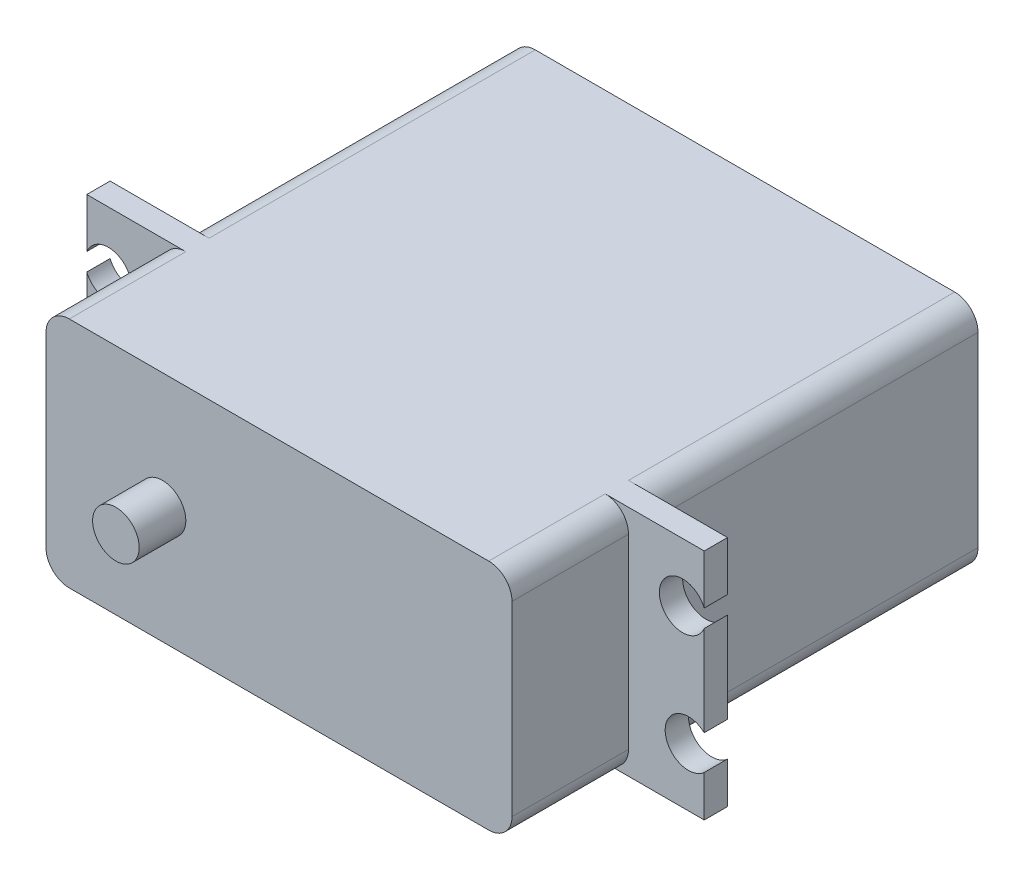
SolidWorks part; units mm, degrees
ref_plane "Front Plane" through (0, 0, 0) normal (0, 0, 1) x (1, 0, 0)
ref_plane "Top Plane" through (0, 0, 0) normal (0, 1, 0) x (1, 0, 0)
ref_plane "Right Plane" through (0, 0, 0) normal (1, 0, 0) x (0, 0, -1)
sketch "Sketch1" plane through (0, 0, 0) normal (0, 1, 0) x (1, 0, 0)
  line L1 (-20, -20) -> (20, -20)
  line L2 (-20, -20) -> (-20, 20)
  line L3 (-20, 20) -> (20, 20)
  line L4 (20, -20) -> (20, 20)
  line L5 (-20, -20) -> (20, 20) construction
  line L6 (-20, 20) -> (20, -20) construction
  point P0 (0, 0)
  dimension "D1" = 40
  dimension "D2" = 40
extrude "Boss-Extrude1" add sketch "Sketch1" along normal blind 20
ref_plane "Plane1" through (0, 0, 8) normal (0, 0, -1) x (-1, 0, 0)
sketch "Sketch2" plane through (0, 0, 8) normal (0, 0, -1) x (-1, 0, 0)
  line L0 (26.5, 0) -> (26.5, 20)
  line L2 (-26.5, 20) -> (-26.5, 0)
  line L4 (-20, 0) -> (20, 0)
  line L5 (20, 0) -> (20, 20)
  line L6 (20, 20) -> (-20, 20)
  line L7 (-20, 20) -> (-20, 0)
  line L8 (-20, 0) -> (20, 0)
  line L9 (20, 0) -> (20, 20)
  line L10 (20, 20) -> (-20, 20)
  line L11 (-20, 20) -> (-20, 0)
  line L12 (20, 0) -> (26.5, 0)
  line L13 (20, 20) -> (26.5, 20)
  line L14 (-20, 0) -> (-26.5, 0)
  line L15 (-20, 20) -> (-26.5, 20)
  line L16 (-26.5, 26.5) -> (-26.5, -6.5) construction
  line L17 (26.5, 26.5) -> (-26.5, 26.5) construction
  line L18 (26.5, -6.5) -> (26.5, 26.5) construction
  line L19 (-26.5, -6.5) -> (26.5, -6.5) construction
  dimension "D1" = 0
  dimension "D2" = 6.5
extrude "Boss-Extrude2" add sketch "Sketch2" against normal blind 2 contours L13 L9 L12 L0 | L11 L15 L2 L14
sketch "Sketch3" plane through (0, 0, 8) normal (0, 0, -1) x (-1, 0, 0)
  line L0 (20, 20) -> (26.5, 20) construction
  line L1 (26.5, 0) -> (26.5, 20) construction
  circle A0 centre (25.1494, 5.0125) radius 2
  circle A1 centre (24.65, 15) radius 2
  dimension "D2" = 4
  dimension "D3" = 4
  dimension "D1" = 10
  dimension "D4" = 5
  dimension "D5" = 1.85
extrude "Cut-Extrude1" cut sketch "Sketch3" against normal blind 2
ref_plane "Plane2" through (0, 0, 0) normal (-1, 0, 0) x (0, 0, 1)
mirror "Mirror2" about plane through (0, 0, 0) normal (-1, 0, 0) of "Cut-Extrude1"
sketch "Sketch4" plane through (0, 0, 20) normal (0, 0, 1) x (1, 0, 0)
  line L0 (20, 20) -> (20, 0) construction
  circle A0 centre (-10, 10) radius 2
  dimension "D2" = 4
  dimension "D1" = 30
extrude "Boss-Extrude3" add sketch "Sketch4" along normal blind 4
fillet "Fillet1" radius 2 8 edges
sketch "Sketch5" plane through (0, 0, 20) normal (0, 0, 1) x (1, 0, 0)
  line L0 (-10, 10) -> (-10, 20) construction
  line L1 (-18, 20) -> (18, 20) construction
sketch "Sketch6" plane through (0, 0, 0) normal (0, 1, 0) x (1, 0, 0)
  line L0 (-10, -20) -> (-10, 20) construction
  line L1 (18, 20) -> (-18, 20) construction
